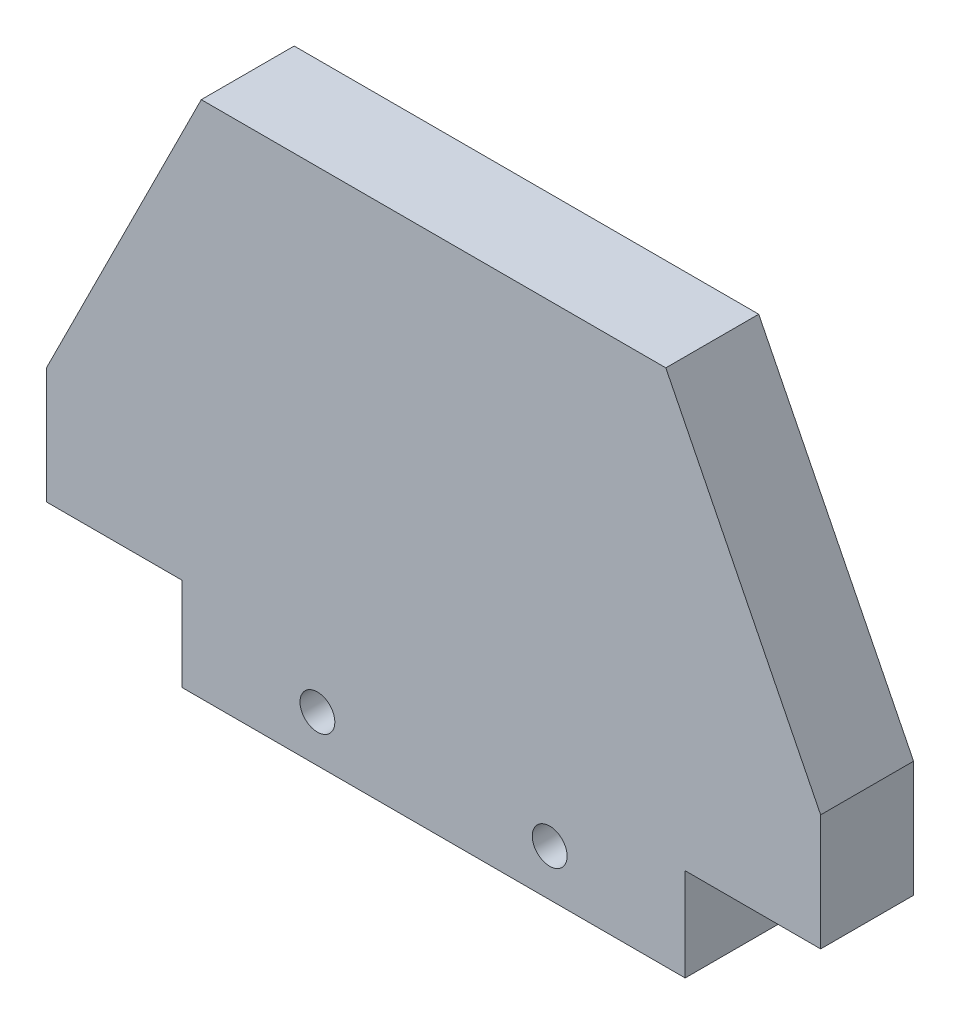
SolidWorks part; units mm, degrees
ref_plane "Front Plane" through (0, 0, 0) normal (0, 0, 1) x (1, 0, 0)
ref_plane "Top Plane" through (0, 0, 0) normal (0, 1, 0) x (1, 0, 0)
ref_plane "Right Plane" through (0, 0, 0) normal (1, 0, 0) x (0, 0, -1)
sketch "Sketch1" plane through (0, 0, 0) normal (0, 0, 1) x (1, 0, 0)
  line L1 (-50, -27.5) -> (50, -27.5)
  line L2 (-50, -27.5) -> (-50, 27.5)
  line L3 (-50, 27.5) -> (50, 27.5)
  line L4 (50, -27.5) -> (50, 27.5)
  line L5 (-50, -27.5) -> (50, 27.5) construction
  line L6 (-50, 27.5) -> (50, -27.5) construction
  point P0 (0, 0)
  dimension "D1" = 100
  dimension "D2" = 55
extrude "Boss-Extrude1" add sketch "Sketch1" along normal blind 12
sketch "Sketch2" plane through (0, -27.5, 0) normal (0, -1, 0) x (1, 0, 0)
  line L0 (-50, 12) -> (50, 12) construction
  line L1 (-32.5, 12) -> (32.5, 12)
  line L2 (-32.5, 12) -> (-32.5, 0)
  line L3 (-32.5, 0) -> (32.5, 0)
  line L4 (32.5, 12) -> (32.5, 0)
  line L5 (-50, 0) -> (50, 0) construction
  line L6 (0, 0) -> (0, 12) construction
  dimension "D1" = 65
extrude "Boss-Extrude2" add sketch "Sketch2" along normal blind 12
hole_wizard "CBORE for M4 Hex Socket Head Cap Screw1" positions "Sketch5" profile "Sketch6" counterbore size "M4" standard "ISO" end condition through all
sketch "Sketch5" plane through (0, 0, 0) normal (0, 0, -1) x (-1, 0, 0)
  line L0 (0, 0) -> (0, -56.9752) construction
  line L2 (32.5, -39.5) -> (-32.5, -39.5) construction
  point P0 (15, -33.5)
  point P2 (-15, -33.5)
  dimension "D1" = 6
  dimension "D2" = 30
sketch "Sketch6" plane through (-15, -33.5, 0) normal (1, 0, 0) x (0, 1, 0)
  line L0 (0, 0) -> (0, 12)
  line L1 (0, 12) -> (2.25, 12)
  line L3 (2.25, 12) -> (2.25, 4.4)
  line L4 (2.25, 4.4) -> (4, 4.4)
  line L5 (4, 4.4) -> (4, 0)
  line L7 (4, 0) -> (0, 0)
  line L11 (0, -6.35) -> (0, 107.95) construction
  dimension "通孔孔直径" = 4.5
  dimension "通孔孔深度" = 12
  dimension "柱形沉头孔直径" = 8
  dimension "柱形沉头孔深度" = 4.4
chamfer "Chamfer1" distance 40 distance2 20 1 edges at (50, 27.5, 6)
chamfer "Chamfer2" distance 20 distance2 40 1 edges at (-50, 27.5, 6)
